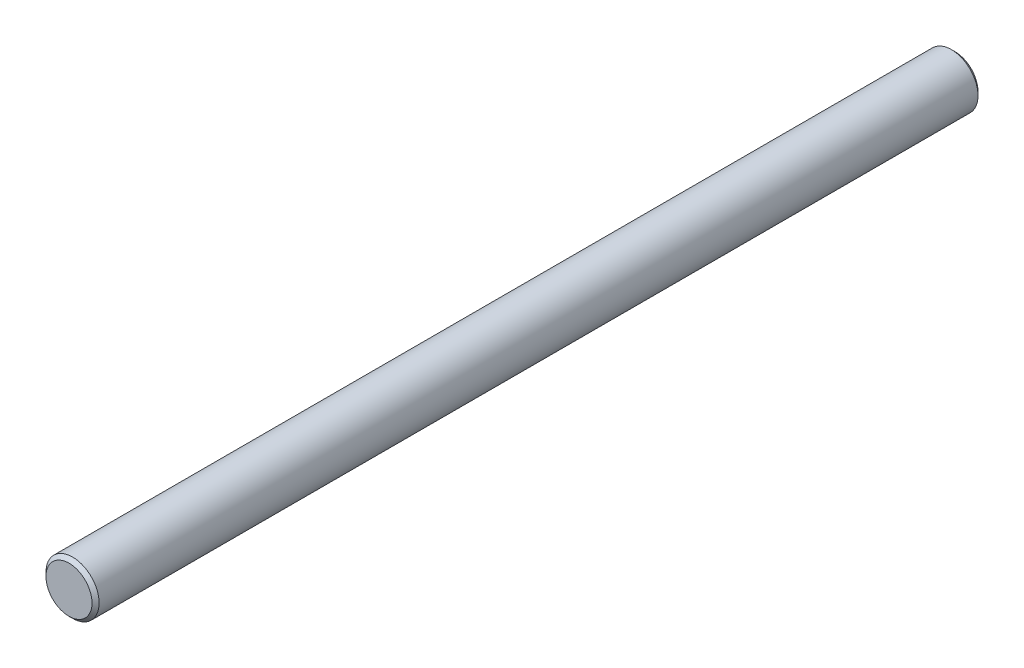
SolidWorks part; units mm, degrees
ref_plane "Front Plane" through (0, 0, 0) normal (0, 0, 1) x (1, 0, 0)
ref_plane "Top Plane" through (0, 0, 0) normal (0, 1, 0) x (1, 0, 0)
ref_plane "Right Plane" through (0, 0, 0) normal (1, 0, 0) x (0, 0, -1)
sketch "Sketch1" plane through (0, 0, 0) normal (0, 0, 1) x (1, 0, 0)
  circle A0 centre (0, 0) radius 0.75
  dimension "D1" = 1.5
extrude "Boss-Extrude1" add sketch "Sketch1" along normal mid plane 25
chamfer "Chamfer1" distance 0.1 angle 45 2 edges at (0.75, 0, -12.5) (0.75, 0, 12.5)
